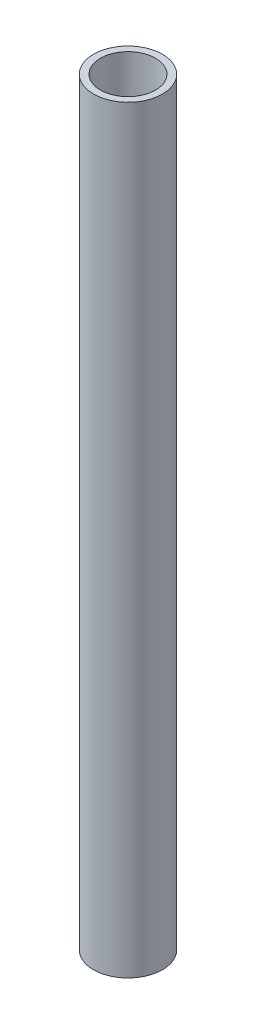
SolidWorks part; units mm, degrees
ref_plane "前视" through (0, 0, 0) normal (0, 0, 1) x (1, 0, 0)
ref_plane "上视" through (0, 0, 0) normal (0, 1, 0) x (1, 0, 0)
ref_plane "右视" through (0, 0, 0) normal (1, 0, 0) x (0, 0, -1)
sketch "草图1" plane through (0, 0, 0) normal (0, 0, 1) x (1, 0, 0)
  line L0 (0, 0) -> (0, 110)
  point P6 (0, 45)
  dimension "D1" = 110
sketch "草图2" plane through (0, 0, 0) normal (0, 1, 0) x (1, 0, 0)
  circle A0 centre (0, 0) radius 5
  circle A1 centre (0, 0) radius 4
  dimension "D1" = 10
  dimension "D2" = 8
sweep "扫描1" add profiles "草图2" path "草图1"
